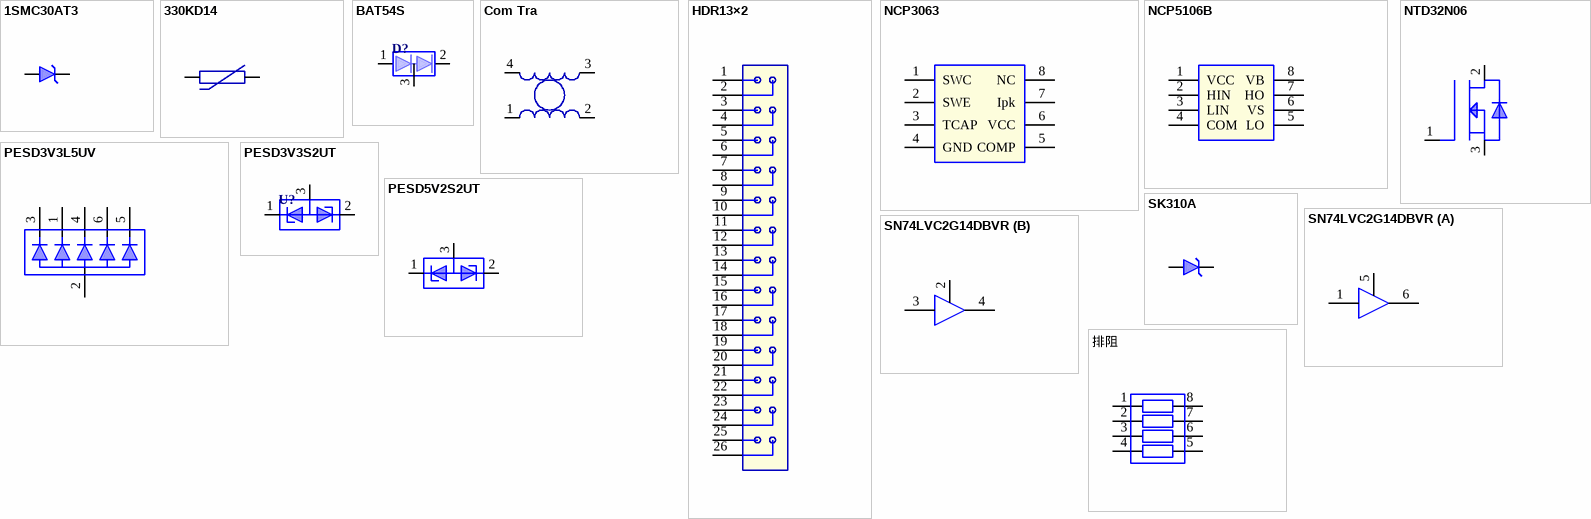
[diagram p0: symbols 1SMC30AT3 to 排阻]
# Altium schematic symbol library MISC103926-16.SchLib: 14 symbols
Pins are listed as number, name and electrical type; pins without a type are passive.


## 1SMC30AT3
designator D?
TVS diode; 名称: MISC103926
footprint Model Name (Footprint not found)
footprint 1SMC17AT
pins: 1, 2
2 alternate drawings of the same symbol

## 330KD14
designator D?
Varistor; 名称: MISC103926
footprint AX-.3/.6
pins: 1, 2
2 alternate drawings of the same symbol

## BAT54S
designator D?
Diode; 名称: MISC103926
footprint SOT-23
pins: 1, 2, 3
2 alternate drawings of the same symbol

## Com Tra
designator T?
Choke coil; 名称: MISC103926
footprint L-2-XIAO
pins: 1, 2, 3, 4
2 alternate drawings of the same symbol

## HDR13×2
designator J?
HDR13×2; 名称: MISC103926
footprint IDC-26
pins: 1, 2, 3, 4, 5, 6, 7, 8, 9, 10, 11, 12, 13, 14, 15, 16, 17, 18, 19, 20, 21, 22, 23, 24, 25, 26
2 alternate drawings of the same symbol

## NCP3063
designator U?
IC; 名称: MISC103926
footprint SO-8
pins: 1 SWC, 2 SWE, 3 TCAP, 4 GND, 5 COMP, 6 VCC, 7 Ipk, 8 NC
2 alternate drawings of the same symbol

## NCP5106B
designator U?
IC; 名称: MISC103926
footprint SO-8
pins: 1 VCC, 2 HIN, 3 LIN, 4 COM, 5 LO, 6 VS, 7 HO, 8 VB
2 alternate drawings of the same symbol

## NTD32N06
designator Q?
MOSFET; 名称: MISC103926
footprint DPAK-3
pins: 1, 2, 3
2 alternate drawings of the same symbol

## PESD3V3L5UV
designator VR?
IC; 名称: MISC103926
footprint SOT666
pins: 1, 2, 3, 4, 5, 6
2 alternate drawings of the same symbol

## PESD3V3S2UT
designator U?
IC; 名称: MISC103926
footprint SOT-23
pins: 1, 2, 3
2 alternate drawings of the same symbol

## PESD5V2S2UT
designator U?
IC; 名称: MISC103926
footprint SOT-23
pins: 1, 2, 3
2 alternate drawings of the same symbol

## SK310A
designator D?
Diode; 名称: MISC103926
footprint DO-214AC
pins: 1, 2
2 alternate drawings of the same symbol

## SN74LVC2G14DBVR
designator U?
IC; 名称: MISC103926
footprint SOT-23-6
part A pins: 1, 5, 6
part B pins: 2, 3, 4
2 alternate drawings of the same symbol

## 排阻
designator RP?
Resistor array; 名称: MISC103926
footprint PZ-4-0.8B
pins: 1, 2, 3, 4, 5, 6, 7, 8
2 alternate drawings of the same symbol